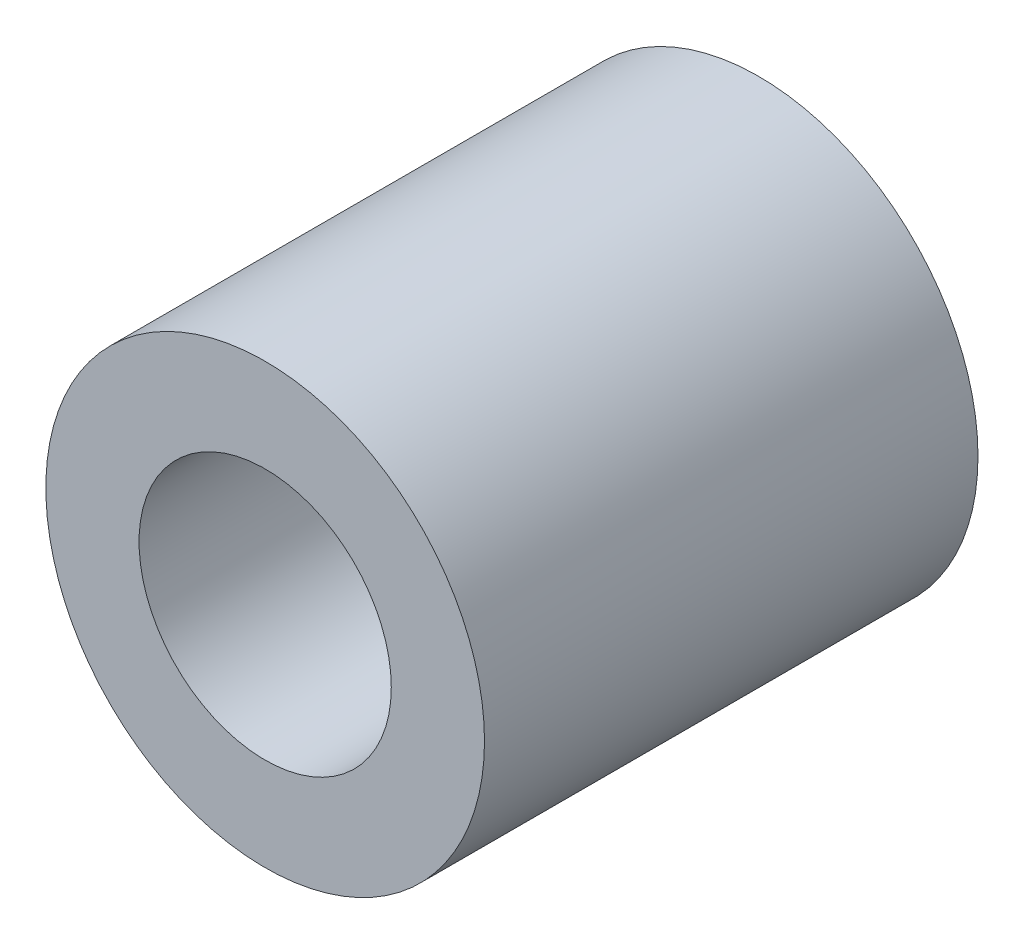
SolidWorks part; units mm, degrees
ref_plane "Front Plane" through (0, 0, 0) normal (0, 0, 1) x (1, 0, 0)
ref_plane "Top Plane" through (0, 0, 0) normal (0, 1, 0) x (1, 0, 0)
ref_plane "Right Plane" through (0, 0, 0) normal (1, 0, 0) x (0, 0, -1)
sketch "Sketch1" plane through (0, 0, 0) normal (0, 0, 1) x (1, 0, 0)
  circle A0 centre (0, 0) radius 2.3
  circle A1 centre (0, 0) radius 4
  dimension "D1" = 4.6
  dimension "D2" = 8
extrude "Boss-Extrude1" add sketch "Sketch1" along normal blind 9
